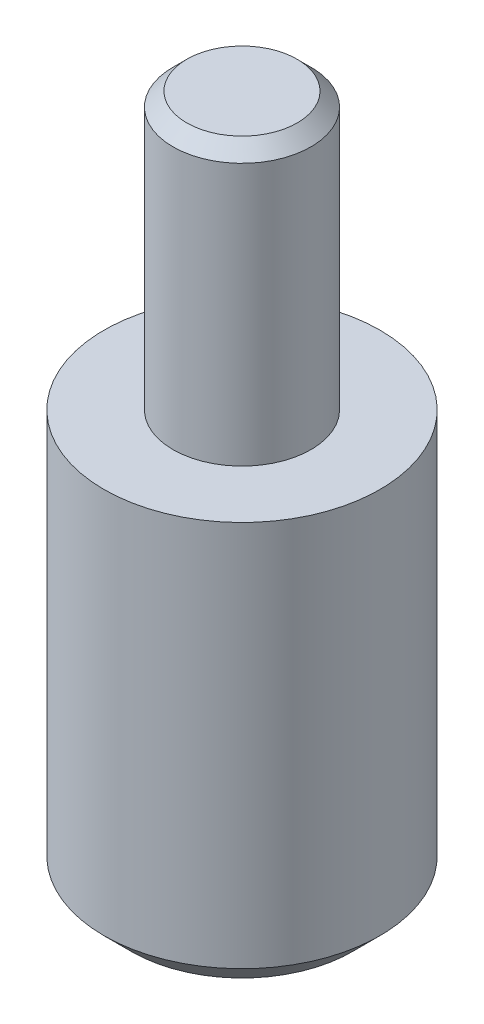
from build123d import *

# Parameters (mm, degrees)
SKETCH1_R           = 10
BOSS_EXTRUDE1_DEPTH = 30
SKETCH2_R           = 5
BOSS_EXTRUDE2_DEPTH = 20
CHAMFER1_SIZE       = 2
CHAMFER2_SIZE       = 1


with BuildPart() as part:
    # Sketch1 → Boss-Extrude1 (new body)
    with BuildSketch(Plane(origin=(0, 0, 0), x_dir=(1, 0, 0), z_dir=(0, 1, 0))):
        with Locations(Location((0, 0, 0), (0, 0, 270))):
            Circle(SKETCH1_R)
    extrude(amount=BOSS_EXTRUDE1_DEPTH)

    # Sketch2 → Boss-Extrude2 (add)
    with BuildSketch(Plane(origin=(0, 30, 0), x_dir=(1, 0, 0), z_dir=(0, 1, 0))):
        with Locations(Location((0, 0, 0), (0, 0, 270))):
            Circle(SKETCH2_R)
    extrude(amount=BOSS_EXTRUDE2_DEPTH)

    # Chamfer1
    chamfer1_edges = [part.edges().sort_by_distance(p)[0] for p in [
        (0, 0, -10),
    ]]
    chamfer(chamfer1_edges, length=CHAMFER1_SIZE)

    # Chamfer2
    chamfer2_edges = [part.edges().sort_by_distance(p)[0] for p in [
        (0, 50, -5),
    ]]
    chamfer(chamfer2_edges, length=CHAMFER2_SIZE)


solid = part.part
